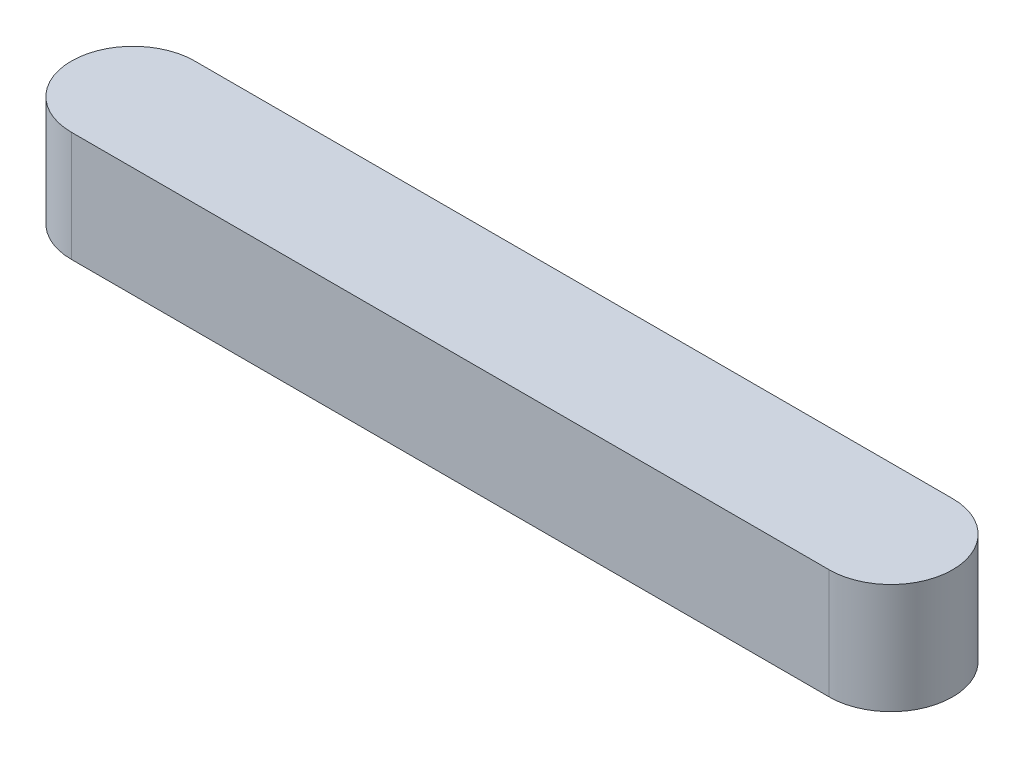
from build123d import *

# Parameters (mm, degrees)
BOSS_EXTRUDE1_DEPTH = 2.5


with BuildPart() as part:
    # Sketch1 → Boss-Extrude1 (new body)
    with BuildSketch(Plane(origin=(0, 0, 0), x_dir=(1, 0, 0), z_dir=(0, 1, 0))):
        with BuildLine():
            Line((-8.6, 1.4), (8.6, 1.4))
            ThreePointArc((8.6, 1.4), (10, 0), (8.6, -1.4))
            Line((8.6, -1.4), (-8.6, -1.4))
            ThreePointArc((-8.6, -1.4), (-10, 0), (-8.6, 1.4))
        make_face()
    extrude(amount=BOSS_EXTRUDE1_DEPTH)


solid = part.part
